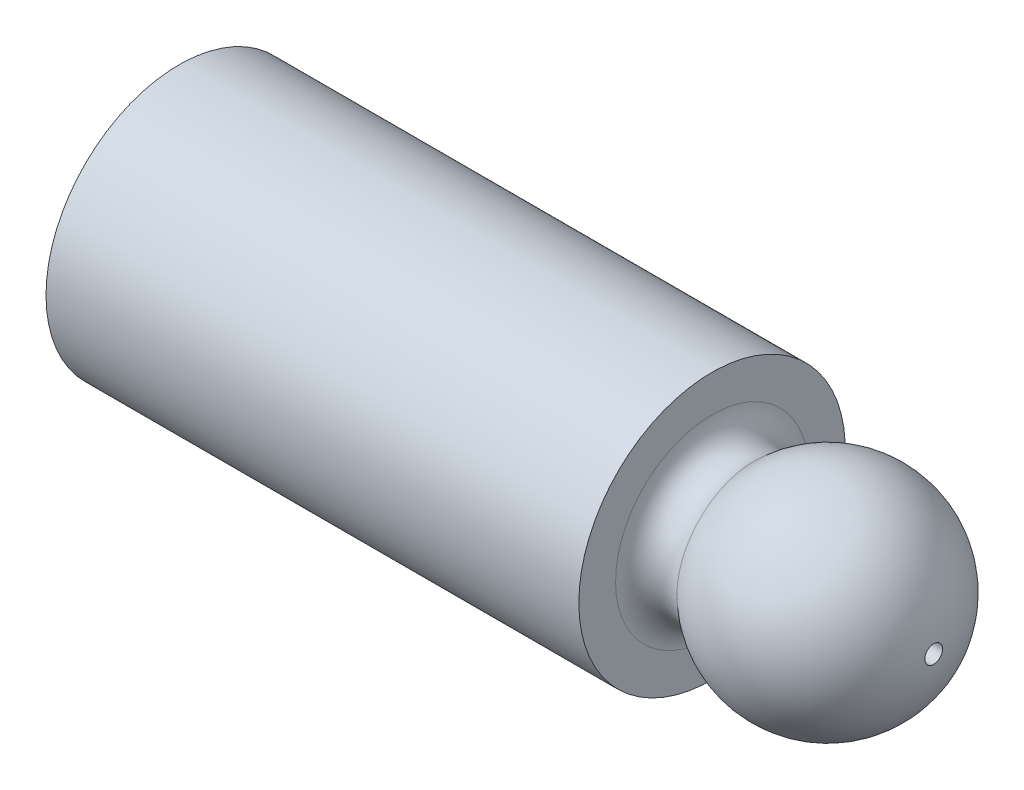
from build123d import *


with BuildPart() as part:
    # Sketch1 → Revolve1 (revolve)
    with BuildSketch(Plane.XY, mode=Mode.PRIVATE) as revolve1_sk:
        with BuildLine():
            Line((0, 0), (0, 7.5))
            Line((0, 7.5), (30, 7.5))
            Line((30, 7.5), (30, 5.431390246))
            ThreePointArc((30, 5.431390246), (30.860121025, 4.119849947), (32.405787349, 4.386048651))
            ThreePointArc((32.405787349, 4.386048651), (38.891100593, 5.502966287), (42.5, 0))
            Line((42.5, 0), (0, 0))
        make_face()
    revolve(revolve1_sk.sketch.rotate(Axis((0, 0, 0), (1, 0, 0)), 90), axis=Axis((0, 0, 0), (1, 0, 0)))

    # Sketch2 → Cut-Revolve1 (revolve, cut)
    with BuildSketch(Plane.XY, mode=Mode.PRIVATE) as cut_revolve1_sk:
        Polygon((0, 0), (25, 0), (27.309401077, 0), (37, 0), (47.95408822, 0), (47.95408822, 0.5), (37, 0.5), (37, 1), (27.309401077, 1), (25, 5), (0, 5), align=None)
    revolve(cut_revolve1_sk.sketch.rotate(Axis((0, 0, 0), (1, 0, 0)), 90), axis=Axis((0, 0, 0), (1, 0, 0)), mode=Mode.SUBTRACT)


solid = part.part
